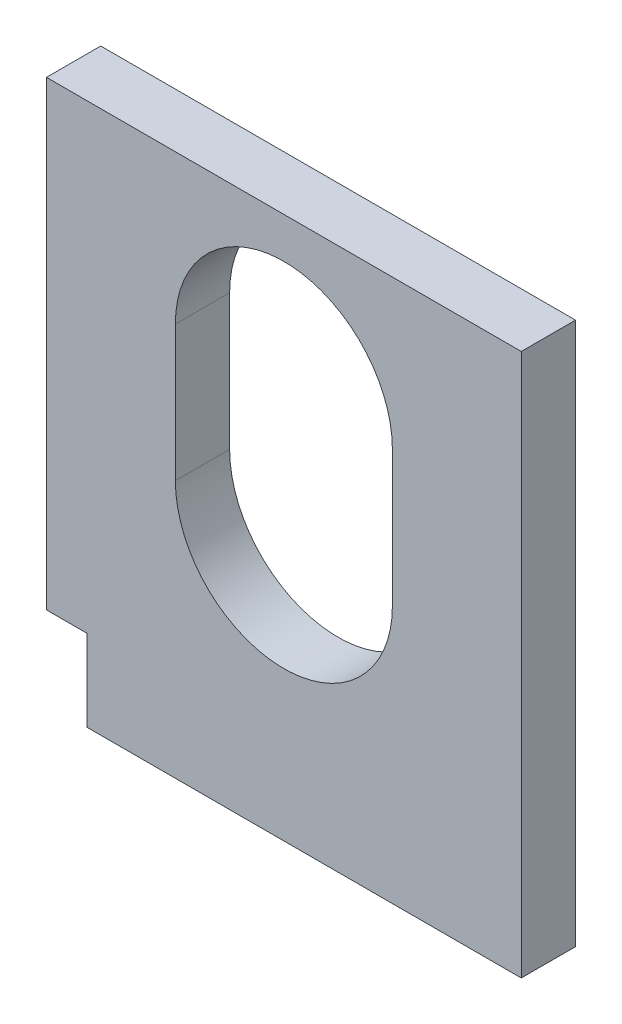
from build123d import *

# Parameters (mm, degrees)
BOSS_EXTRUDE1_DEPTH = 4


with BuildPart() as part:
    # Sketch1 → Boss-Extrude1 (new body)
    with BuildSketch(Plane.XY):
        Polygon((3, 0), (35, 0), (35, 40), (0, 40), (0, 5.997826072), (3, 5.997826072), align=None)
        with BuildLine():
            Line((9.5, 29), (9.5, 19))
            ThreePointArc((9.5, 19), (17.5, 11), (25.5, 19))
            Line((25.5, 19), (25.5, 29))
            ThreePointArc((25.5, 29), (17.5, 37), (9.5, 29))
        make_face(mode=Mode.SUBTRACT)
    extrude(amount=BOSS_EXTRUDE1_DEPTH)


solid = part.part
